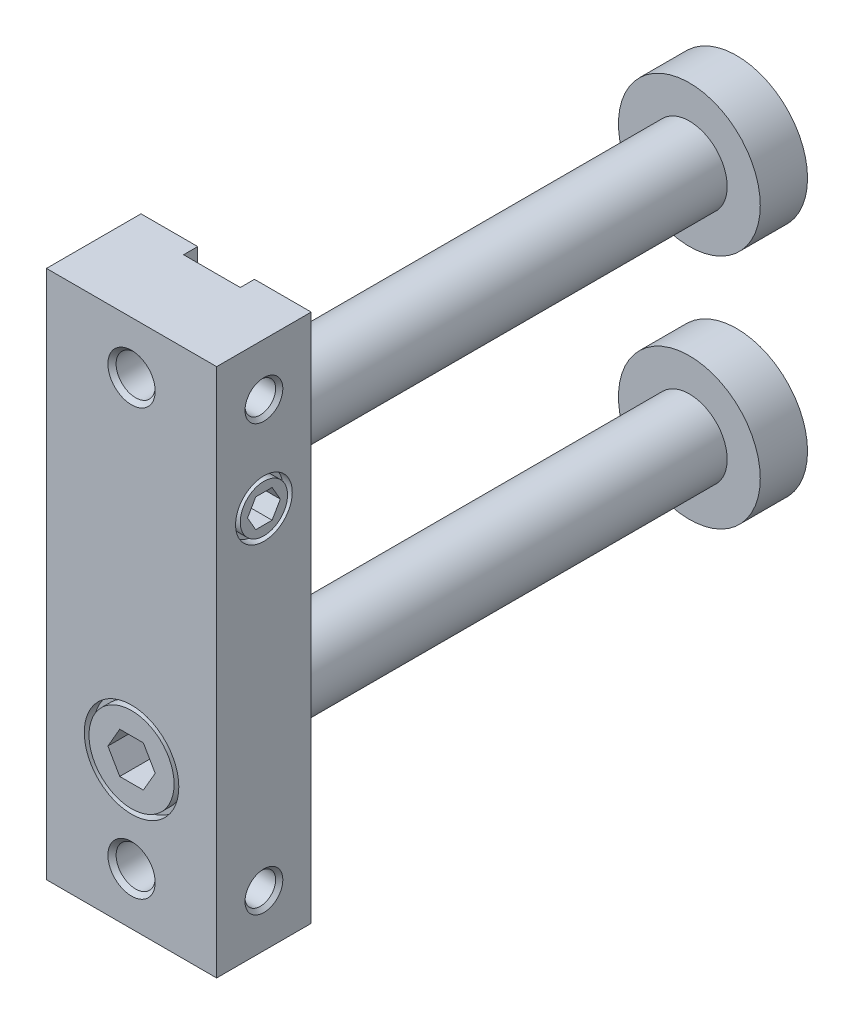
from build123d import *

# Parameters (mm, degrees)
SKETCH1_W           = 18
SKETCH1_H           = 56
BOSS_EXTRUDE1_DEPTH = 10
SKETCH2_W           = 6
SKETCH2_H           = 56
CUT_EXTRUDE1_DEPTH  = 1.5
HOLE1_D             = 3.242
HOLE1_DEPTH         = 6
HOLE1_CSINK_D       = 4
HOLE1_CSINK_ANGLE   = 90
HOLE1_TIP           = 0.935884786
HOLE2_D             = 3.242
HOLE2_DEPTH         = 6
HOLE2_CSINK_D       = 4
HOLE2_CSINK_ANGLE   = 90
HOLE2_TIP           = 0.935884786
HOLE3_D             = 3.242
HOLE3_DEPTH         = 6
HOLE3_CSINK_D       = 4
HOLE3_CSINK_ANGLE   = 90
HOLE3_TIP           = 0.935884786
HOLE4_D             = 3.242
HOLE4_DEPTH         = 6
HOLE4_CSINK_D       = 4
HOLE4_CSINK_ANGLE   = 90
HOLE4_TIP           = 0.935884786
SKETCH15_R          = 5
SKETCH15_R_2        = 4.5
CUT_EXTRUDE2_DEPTH  = 1
CUT_EXTRUDE3_DEPTH  = 4.33
SKETCH17_R          = 3
SKETCH17_R_2        = 2.5
CUT_EXTRUDE4_DEPTH  = 1
CUT_EXTRUDE5_DEPTH  = 3


with BuildPart() as part:
    # Sketch1 → Boss-Extrude1 (new body)
    with BuildSketch(Plane.XY.offset(9)):
        Rectangle(SKETCH1_W, SKETCH1_H)
    extrude(amount=BOSS_EXTRUDE1_DEPTH)

    # Sketch2 → Cut-Extrude1 (cut)
    with BuildSketch(Plane.XY.offset(9)):
        Rectangle(SKETCH2_W, SKETCH2_H)
    extrude(amount=CUT_EXTRUDE1_DEPTH, mode=Mode.SUBTRACT)

    # Sketch3 → Revolve1 (revolve)
    with BuildSketch(Plane(origin=(0, 0, 0), x_dir=(0, 0, -1), z_dir=(1, 0, 0)), mode=Mode.PRIVATE) as revolve1_sk:
        Polygon((-14, 12.5), (-14, 16.5), (40, 16.5), (40, 20), (45, 20), (45, 12.5), align=None)
    revolve(revolve1_sk.sketch.rotate(Axis((0, 12.5, -45), (0, 0, 1)), 270), axis=Axis((0, 12.5, -45), (0, 0, 1)))

    # Sketch4 → Revolve2 (revolve)
    with BuildSketch(Plane(origin=(0, 0, 0), x_dir=(0, 0, -1), z_dir=(1, 0, 0)), mode=Mode.PRIVATE) as revolve2_sk:
        Polygon((-14, -12.5), (-14, -8.5), (40, -8.5), (40, -5), (45, -5), (45, -12.5), align=None)
    revolve(revolve2_sk.sketch.rotate(Axis((0, -12.5, -45), (0, 0, 1)), 270), axis=Axis((0, -12.5, -45), (0, 0, 1)))

    # Sketch5 → Cut-Revolve1 (revolve, cut)
    with BuildSketch(Plane(origin=(0, 0, 0), x_dir=(0, 0, -1), z_dir=(1, 0, 0)), mode=Mode.PRIVATE) as cut_revolve1_sk:
        Polygon((-19, 22.5), (-19, 25), (-18.567, 24.567), (-10.933, 24.567), (-10.5, 25), (-10.5, 22.5), align=None)
    revolve(cut_revolve1_sk.sketch.rotate(Axis((0, 22.5, 10.5), (0, 0, 1)), 270), axis=Axis((0, 22.5, 10.5), (0, 0, 1)), mode=Mode.SUBTRACT)

    # Sketch6 → Cut-Revolve2 (revolve, cut)
    with BuildSketch(Plane(origin=(0, 0, 0), x_dir=(0, 0, -1), z_dir=(1, 0, 0)), mode=Mode.PRIVATE) as cut_revolve2_sk:
        Polygon((-19, -22.5), (-19, -20), (-18.567, -20.433), (-10.933, -20.433), (-10.5, -20), (-10.5, -22.5), align=None)
    revolve(cut_revolve2_sk.sketch.rotate(Axis((0, -22.5, 10.5), (0, 0, 1)), 270), axis=Axis((0, -22.5, 10.5), (0, 0, 1)), mode=Mode.SUBTRACT)

    # Hole1
    with Locations(Plane.ZY.offset(9)):
        with Locations((14, 22.5)):
            CounterSinkHole(HOLE1_D / 2, HOLE1_CSINK_D / 2, depth=HOLE1_DEPTH, counter_sink_angle=HOLE1_CSINK_ANGLE)
            with Locations((0, 0, -(HOLE1_DEPTH + HOLE1_TIP / 2))):  # 120° drill point
                Cone(0, HOLE1_D / 2, HOLE1_TIP, mode=Mode.SUBTRACT)

    # Hole2
    with Locations(Plane.ZY.offset(9)):
        with Locations((14, -22.5)):
            CounterSinkHole(HOLE2_D / 2, HOLE2_CSINK_D / 2, depth=HOLE2_DEPTH, counter_sink_angle=HOLE2_CSINK_ANGLE)
            with Locations((0, 0, -(HOLE2_DEPTH + HOLE2_TIP / 2))):  # 120° drill point
                Cone(0, HOLE2_D / 2, HOLE2_TIP, mode=Mode.SUBTRACT)

    # Hole3
    with Locations(Plane(origin=(9, 0, 0), x_dir=(0, 0, -1), z_dir=(1, 0, 0))):
        with Locations((-14, 22.5)):
            CounterSinkHole(HOLE3_D / 2, HOLE3_CSINK_D / 2, depth=HOLE3_DEPTH, counter_sink_angle=HOLE3_CSINK_ANGLE)
            with Locations((0, 0, -(HOLE3_DEPTH + HOLE3_TIP / 2))):  # 120° drill point
                Cone(0, HOLE3_D / 2, HOLE3_TIP, mode=Mode.SUBTRACT)

    # Hole4
    with Locations(Plane(origin=(9, 0, 0), x_dir=(0, 0, -1), z_dir=(1, 0, 0))):
        with Locations((-14, -22.5)):
            CounterSinkHole(HOLE4_D / 2, HOLE4_CSINK_D / 2, depth=HOLE4_DEPTH, counter_sink_angle=HOLE4_CSINK_ANGLE)
            with Locations((0, 0, -(HOLE4_DEPTH + HOLE4_TIP / 2))):  # 120° drill point
                Cone(0, HOLE4_D / 2, HOLE4_TIP, mode=Mode.SUBTRACT)

    # Sketch15 → Cut-Extrude2 (cut)
    with BuildSketch(Plane.XY.offset(19)):
        with Locations((0, -12.5)):
            Circle(SKETCH15_R)
        with Locations((0, -12.5)):
            Circle(SKETCH15_R_2, mode=Mode.SUBTRACT)
    extrude(amount=-CUT_EXTRUDE2_DEPTH, mode=Mode.SUBTRACT)

    # Sketch16 → Cut-Extrude3 (cut)
    with BuildSketch(Plane.XY.offset(19)):
        Polygon((-2.499926666, -12.5), (-1.249963333, -14.665), (1.249963333, -14.665), (2.499926666, -12.5), (1.249963333, -10.335), (-1.249963333, -10.335), align=None)
    extrude(amount=-CUT_EXTRUDE3_DEPTH, mode=Mode.SUBTRACT)

    # Sketch17 → Cut-Extrude4 (cut)
    with BuildSketch(Plane(origin=(9, 0, 0), x_dir=(0, 0, -1), z_dir=(1, 0, 0))):
        with Locations((-14, 12.5)):
            Circle(SKETCH17_R)
        with Locations((-14, 12.5)):
            Circle(SKETCH17_R_2, mode=Mode.SUBTRACT)
    extrude(amount=-CUT_EXTRUDE4_DEPTH, mode=Mode.SUBTRACT)

    # Sketch18 → Cut-Extrude5 (cut)
    with BuildSketch(Plane(origin=(9, 0, 0), x_dir=(0, 0, -1), z_dir=(1, 0, 0))):
        Polygon((-15.732050808, 12.5), (-14.866025404, 11), (-13.133974596, 11), (-12.267949192, 12.5), (-13.133974596, 14), (-14.866025404, 14), align=None)
    extrude(amount=-CUT_EXTRUDE5_DEPTH, mode=Mode.SUBTRACT)


solid = part.part
